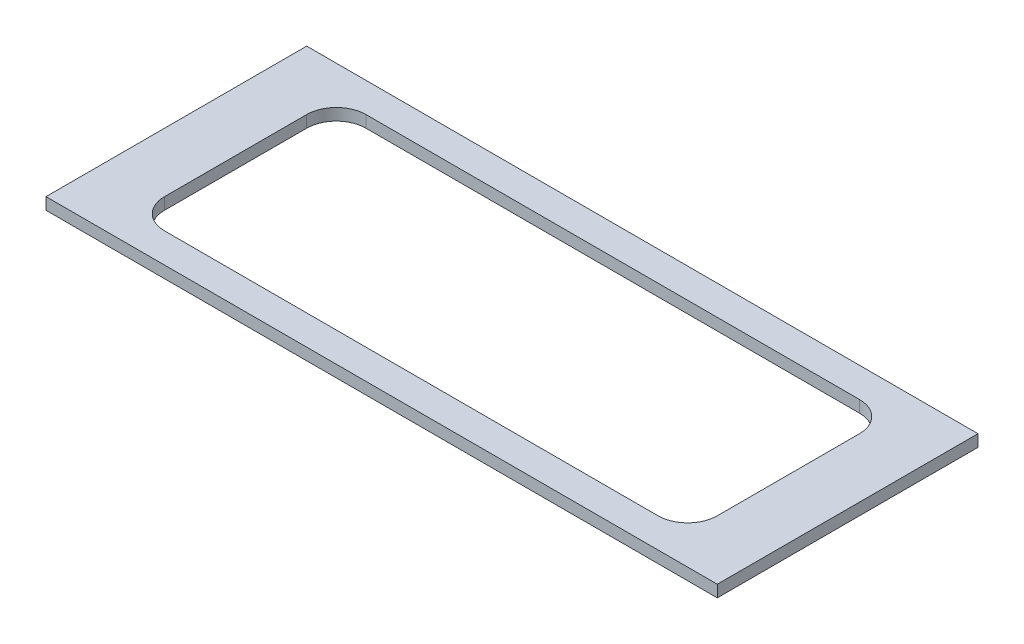
from build123d import *

# Parameters (mm, degrees)
SKETCH_1_W          = 2266
SKETCH_1_H          = 880
EXTRUDE_1_DEPTH     = 40
SKETCH_2_W          = 1866
SKETCH_2_H          = 680
CUT_EXTRUDE_1_DEPTH = 1217.095802147
FILLET_1_R          = 100


with BuildPart() as part:
    # 草图1 → 凸台-拉伸1 (new body)
    with BuildSketch(Plane(origin=(0, 0, 0), x_dir=(1, 0, 0), z_dir=(0, 1, 0))):
        Rectangle(SKETCH_1_W, SKETCH_1_H)
    extrude(amount=EXTRUDE_1_DEPTH)

    # 草图2 → 切除-拉伸1 (cut, through all)
    with BuildSketch(Plane.XZ):
        Rectangle(SKETCH_2_W, SKETCH_2_H)
    extrude(amount=-CUT_EXTRUDE_1_DEPTH, mode=Mode.SUBTRACT)

    # 圆角1
    fillet_1_edges = [part.edges().sort_by_distance(p)[0] for p in [
        (933, 20, 340),
        (933, 20, -340),
        (-933, 20, -340),
        (-933, 20, 340),
    ]]
    fillet(fillet_1_edges, radius=FILLET_1_R)


solid = part.part
